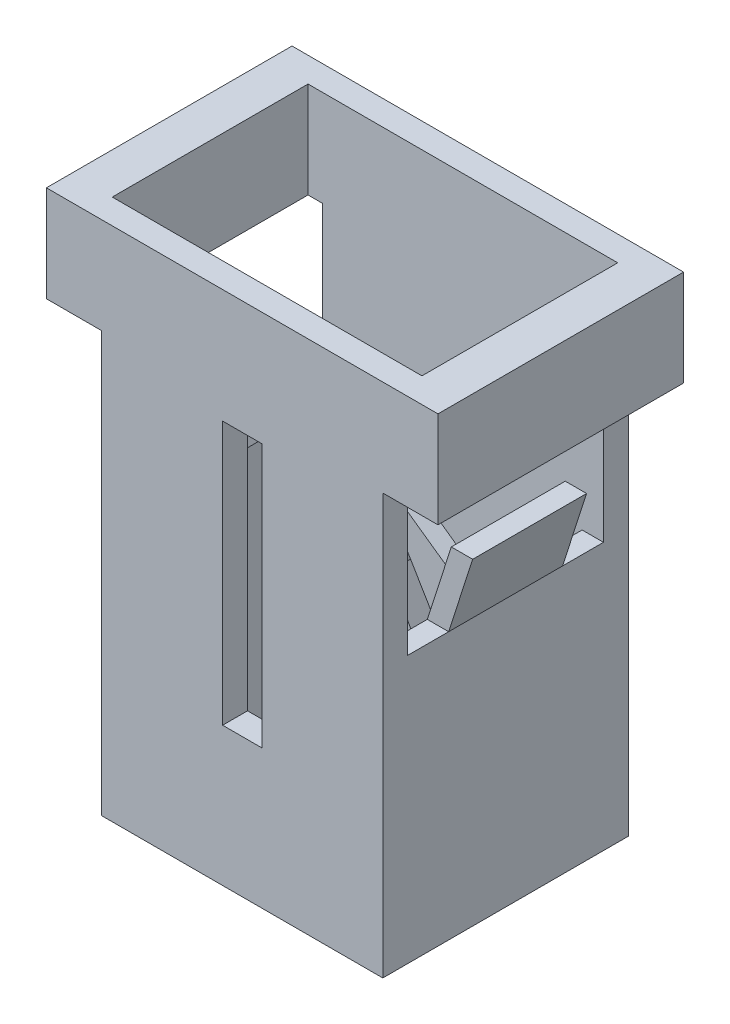
from build123d import *

# Parameters (mm, degrees)
EXTRUDE_1_DEPTH     = 3.45
CHAMFER_1_SIZE      = 0.5
SKETCH_2_W          = 5.5
SKETCH_2_H          = 4.3
CUT_EXTRUDE_1_DEPTH = 19.061146143
SKETCH_3_W          = 8.7
SKETCH_3_H          = 5.5
CUT_EXTRUDE_2_DEPTH = 2.7
SKETCH_5_W          = 6.7
SKETCH_5_H          = 5.5
CUT_EXTRUDE_3_DEPTH = 14
SKETCH_6_W          = 1.1
SKETCH_6_H          = 7.4
CUT_EXTRUDE_4_DEPTH = 1
EXTRUDE_2_DEPTH     = 1.6
SKETCH_8_W          = 2
SKETCH_8_H          = 1
CUT_EXTRUDE_5_DEPTH = 3.5
SKETCH_9_R          = 0.75
EXTRUDE_3_DEPTH     = 3.2
DRAFT_1_ANGLE       = 2
CUT_EXTRUDE_6_DEPTH = 3.2
EXTRUDE_4_DEPTH     = 0.5
SCALE_1_SCALE       = 0.7


with BuildPart() as part:
    # 草图1 → 凸台-拉伸1 (new, symmetric)
    with BuildSketch(Plane.XY):
        Polygon((-3.95, 0), (3.95, 0), (3.95, 12.3), (5.5, 12.3), (5.5, 15), (-5.5, 15), (-5.5, 12.3), (-3.95, 12.3), align=None)
    extrude(amount=EXTRUDE_1_DEPTH, both=True)

    # 倒角1
    chamfer_1_edges = [part.edges().sort_by_distance(p)[0] for p in [
        (3.95, 0, 0),
        (-3.95, 0, 0),
        (0, 0, 3.45),
        (0, 0, -3.45),
    ]]
    chamfer(chamfer_1_edges, length=CHAMFER_1_SIZE)

    # 草图2 → 切除-拉伸1 (cut, through all)
    with BuildSketch(Plane.ZY.offset(3.95)):
        with Locations((0, 10.15)):
            Rectangle(SKETCH_2_W, SKETCH_2_H)
    extrude(amount=-CUT_EXTRUDE_1_DEPTH, mode=Mode.SUBTRACT)

    # 草图3 → 切除-拉伸2 (cut)
    with BuildSketch(Plane(origin=(0, 15, 0), x_dir=(1, 0, 0), z_dir=(0, 1, 0))):
        Rectangle(SKETCH_3_W, SKETCH_3_H)
    extrude(amount=-CUT_EXTRUDE_2_DEPTH, mode=Mode.SUBTRACT)

    # 草图5 → 切除-拉伸3 (cut)
    with BuildSketch(Plane(origin=(0, 15, 0), x_dir=(1, 0, 0), z_dir=(0, 1, 0))):
        Rectangle(SKETCH_5_W, SKETCH_5_H)
    extrude(amount=-CUT_EXTRUDE_3_DEPTH, mode=Mode.SUBTRACT)

    # 草图6 → 切除-拉伸4 (cut)
    with BuildSketch(Plane.XY.offset(3.45)):
        with Locations((0, 8.1)):
            Rectangle(SKETCH_6_W, SKETCH_6_H)
    extrude(amount=-CUT_EXTRUDE_4_DEPTH, mode=Mode.SUBTRACT)

    # 草图7 → 凸台-拉伸2 (add, symmetric)
    with BuildSketch(Plane.XY):
        Polygon((-3.95, 8), (-4.625, 10.1), (-4.025, 10.1), (-3.35, 8), align=None)
        Polygon((3.35, 8), (3.95, 8), (4.625, 10.1), (4.025, 10.1), align=None)
    extrude(amount=EXTRUDE_2_DEPTH, both=True)

    # 草图8 → 切除-拉伸5 (cut)
    with BuildSketch(Plane.XZ):
        with Locations((-1.55, -1.75)):
            Rectangle(SKETCH_8_W, SKETCH_8_H)
        with Locations((1.55, -1.75)):
            Rectangle(SKETCH_8_W, SKETCH_8_H)
    extrude(amount=-CUT_EXTRUDE_5_DEPTH, mode=Mode.SUBTRACT)

    # 草图9 → 凸台-拉伸3 (add)
    with BuildSketch(Plane(origin=(0, 1, 0), x_dir=(1, 0, 0), z_dir=(0, 1, 0))):
        with Locations(Location((0, -0.55, 0), (0, 0, 270))):
            Circle(SKETCH_9_R)
    extrude(amount=EXTRUDE_3_DEPTH)

    # 拔模1
    draft_1_faces = [part.faces().sort_by_distance(p)[0] for p in [
        (0, 2.6, -0.2),
    ]]
    draft(draft_1_faces, Plane.ZX.offset(1), DRAFT_1_ANGLE)

    # 草图10 → 切除-拉伸6 (cut)
    with BuildSketch(Plane(origin=(0, 0, -3.45), x_dir=(-1, 0, 0), z_dir=(0, 0, -1))):
        Polygon((-2.05, 4.3), (-2.05, 2.7), (-1.15, 3.1), (-0.2, 2.4), (1.05, 2.4), (2.05, 4.3), (2.05, 7.2), (0.15, 4), (-0.55, 4.6), align=None)
    extrude(amount=-CUT_EXTRUDE_6_DEPTH, mode=Mode.SUBTRACT)

    # 草图11 → 凸台-拉伸4 (add)
    with BuildSketch(Plane.XY.offset(-2.75)):
        Polygon((0.55, 4.6), (2.05, 4.3), (-2.05, 7.2), (-0.15, 4), align=None)
    extrude(amount=EXTRUDE_4_DEPTH)


with BuildPart() as part_1:
    # 缩放比例1: scaled about (0.005424554, 7.149122165, 0.023385792)
    add(part.part.scale(SCALE_1_SCALE).moved(Location((0.001627366, 2.14473665, 0.007015738))))


solid = part_1.part
